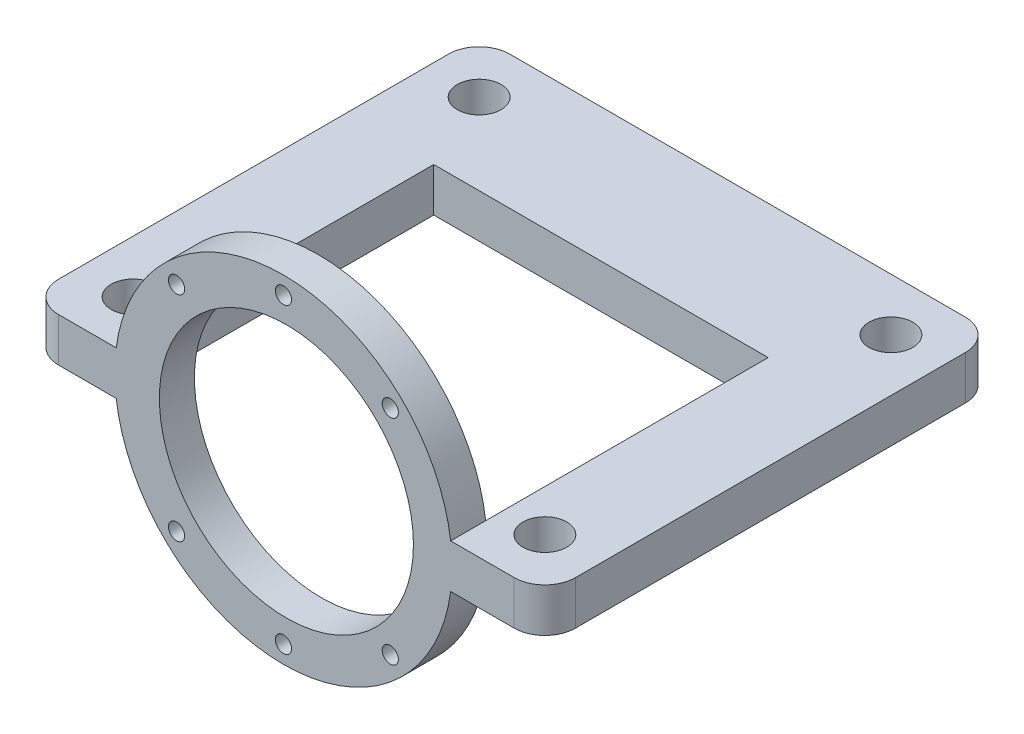
from build123d import *

# Parameters (mm, degrees)
SKETCH2_R                = 38.5
SKETCH2_R_2              = 29
SKETCH2_R_3              = 1.85
BOSS_EXTRUDE1_DEPTH      = 8
BOSS_EXTRUDE2_DEPTH      = 5
BOSS_EXTRUDE2_DEPTH_BACK = 5
SKETCH4_W                = 22.91440569
SKETCH4_H                = 10
SKETCH4_W_2              = 25.697687416
BOSS_EXTRUDE3_DEPTH      = 8
CUT_EXTRUDE1_REACH       = 122.328
SKETCH5_R                = 5
FILLET1_R                = 7
CUT_EXTRUDE2_REACH       = 122.328
SKETCH6_W                = 76.347887986
SKETCH6_H                = 64.488526755


with BuildPart() as part:
    # Sketch2 → Boss-Extrude1 (new body)
    with BuildSketch(Plane.XY):
        Circle(SKETCH2_R)
        with Locations((0.678631435, 0)):
            Circle(SKETCH2_R_2, mode=Mode.SUBTRACT)
        with Locations((0, 34.5)):
            Circle(SKETCH2_R_3, mode=Mode.SUBTRACT)
        with Locations((24.395183951, 24.395183951)):
            Circle(SKETCH2_R_3, mode=Mode.SUBTRACT)
        with Locations((24.395183951, -24.395183951)):
            Circle(SKETCH2_R_3, mode=Mode.SUBTRACT)
        with Locations((0, -34.5)):
            Circle(SKETCH2_R_3, mode=Mode.SUBTRACT)
        with Locations((-24.395183951, -24.395183951)):
            Circle(SKETCH2_R_3, mode=Mode.SUBTRACT)
        with Locations((-24.395183951, 24.395183951)):
            Circle(SKETCH2_R_3, mode=Mode.SUBTRACT)
    extrude(amount=BOSS_EXTRUDE1_DEPTH)

    # Sketch3 → Boss-Extrude2 (add, two sides: drawn at the far end of the back side and taken through both)
    with BuildSketch(Plane(origin=(0, 0, 0), x_dir=(1, 0, 0), z_dir=(0, 1, 0)).offset(-BOSS_EXTRUDE2_DEPTH_BACK)):
        Polygon((-28.321368565, 0), (-38.5, 0), (-58.321368565, 0), (-58.321368565, 67.772616809), (-58.321368565, 95), (59.678631435, 95), (59.678631435, 67.772616809), (59.678631435, 0), (38.5, 0), (29.678631435, 0), (29.678631435, 60), (-28.321368565, 60), align=None)
    extrude(amount=BOSS_EXTRUDE2_DEPTH + BOSS_EXTRUDE2_DEPTH_BACK)

    # Sketch4 → Boss-Extrude3 (add)
    with BuildSketch(Plane.XY):
        with Locations((-46.86416572, 0)):
            Rectangle(SKETCH4_W, SKETCH4_H)
        with Locations((46.829787727, 0)):
            Rectangle(SKETCH4_W_2, SKETCH4_H)
    extrude(amount=BOSS_EXTRUDE3_DEPTH)

    # Sketch5 → Cut-Extrude1 (cut, up to next)
    with BuildSketch(Plane(origin=(0, 5, 0), x_dir=(1, 0, 0), z_dir=(0, 1, 0)), mode=Mode.PRIVATE) as cut_extrude1_sk1:
        with Locations(Location((-46.321368565, 83, 0), (0, 0, 270))):
            Circle(SKETCH5_R)
    cut_extrude1_tool1 = extrude(cut_extrude1_sk1.sketch, amount=-CUT_EXTRUDE1_REACH, mode=Mode.PRIVATE) & part.part
    # Sketch5 → Cut-Extrude1 (cut, up to next)
    with BuildSketch(Plane(origin=(0, 5, 0), x_dir=(1, 0, 0), z_dir=(0, 1, 0)), mode=Mode.PRIVATE) as cut_extrude1_sk2:
        with Locations(Location((-46.321368565, 4, 0), (0, 0, 270))):
            Circle(SKETCH5_R)
    cut_extrude1_tool2 = extrude(cut_extrude1_sk2.sketch, amount=-CUT_EXTRUDE1_REACH, mode=Mode.PRIVATE) & part.part
    # Sketch5 → Cut-Extrude1 (cut, up to next)
    with BuildSketch(Plane(origin=(0, 5, 0), x_dir=(1, 0, 0), z_dir=(0, 1, 0)), mode=Mode.PRIVATE) as cut_extrude1_sk3:
        with Locations(Location((47.678631435, 83, 0), (0, 0, 270))):
            Circle(SKETCH5_R)
    cut_extrude1_tool3 = extrude(cut_extrude1_sk3.sketch, amount=-CUT_EXTRUDE1_REACH, mode=Mode.PRIVATE) & part.part
    # Sketch5 → Cut-Extrude1 (cut, up to next)
    with BuildSketch(Plane(origin=(0, 5, 0), x_dir=(1, 0, 0), z_dir=(0, 1, 0)), mode=Mode.PRIVATE) as cut_extrude1_sk4:
        with Locations(Location((47.678631435, 4, 0), (0, 0, 270))):
            Circle(SKETCH5_R)
    cut_extrude1_tool4 = extrude(cut_extrude1_sk4.sketch, amount=-CUT_EXTRUDE1_REACH, mode=Mode.PRIVATE) & part.part
    add(cut_extrude1_tool1.solids().sort_by_distance((-46.321369, 5, -83))[0], mode=Mode.SUBTRACT)
    add(cut_extrude1_tool2.solids().sort_by_distance((-46.321369, 5, -4))[0], mode=Mode.SUBTRACT)
    add(cut_extrude1_tool3.solids().sort_by_distance((47.678631, 5, -83))[0], mode=Mode.SUBTRACT)
    add(cut_extrude1_tool4.solids().sort_by_distance((47.678631, 5, -4))[0], mode=Mode.SUBTRACT)

    # Fillet1
    fillet1_edges = [part.edges().sort_by_distance(p)[0] for p in [
        (-28.321368565, 0, -60),
        (-58.321368565, 0, -95),
        (59.678631435, 0, -95),
        (29.678631435, 0, -60),
        (-58.321368565, 0, 8),
        (59.678631435, 0, 8),
    ]]
    fillet(fillet1_edges, radius=FILLET1_R)

    # Sketch6 → Cut-Extrude2 (cut, up to next)
    with BuildSketch(Plane(origin=(0, 5, 0), x_dir=(1, 0, 0), z_dir=(0, 1, 0)), mode=Mode.PRIVATE) as cut_extrude2_sk1:
        with Locations((0, 32.244263378)):
            Rectangle(SKETCH6_W, SKETCH6_H)
    cut_extrude2_tool1 = extrude(cut_extrude2_sk1.sketch, amount=-CUT_EXTRUDE2_REACH, mode=Mode.PRIVATE) & part.part
    add(cut_extrude2_tool1.solids().sort_by_distance((0, 5, -32.244263))[0], mode=Mode.SUBTRACT)


solid = part.part
